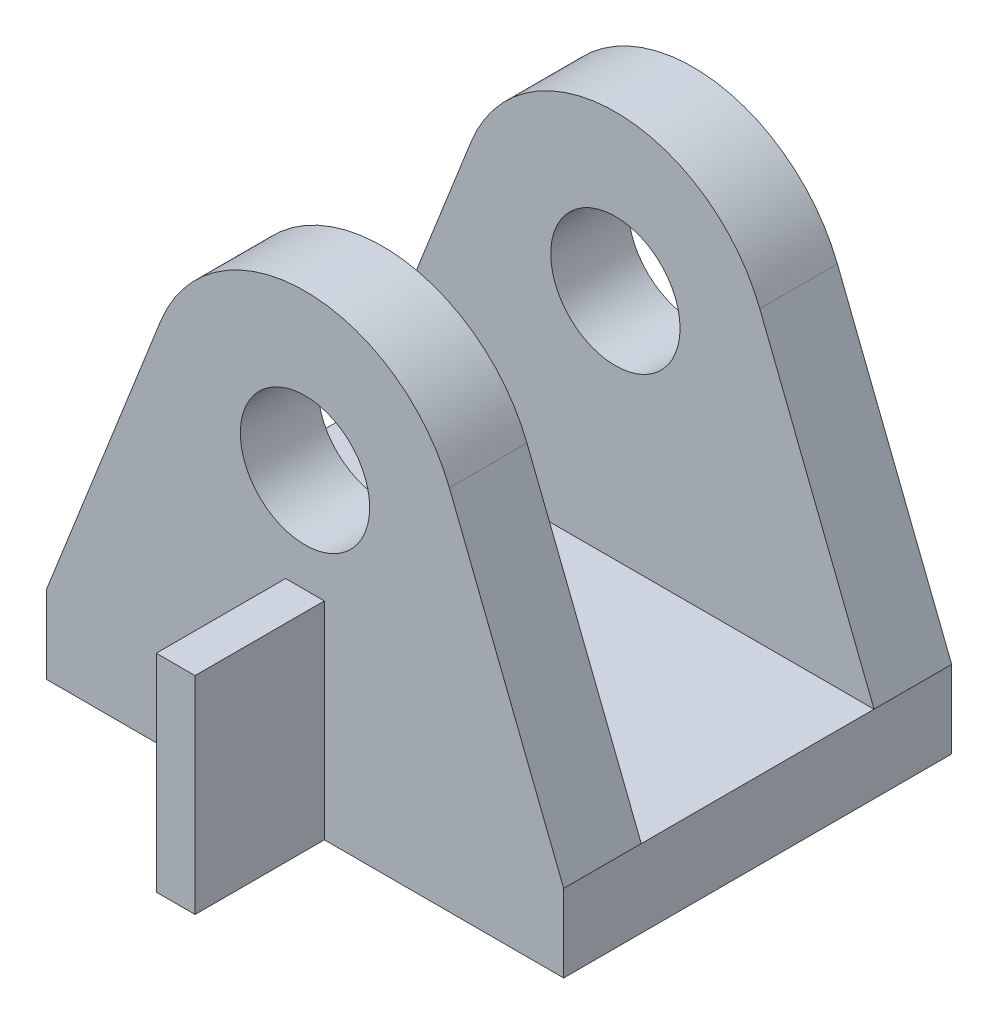
from build123d import *

# Parameters (mm, degrees)
SKETCH_1_W           = 200
SKETCH_1_H           = 150
BOSS_EXTRUDE_1_DEPTH = 30
SKETCH_2_R           = 25
BOSS_EXTRUDE_2_DEPTH = 30
SKETCH_4_W           = 15
SKETCH_4_H           = 80
BOSS_EXTRUDE_3_DEPTH = 50


with BuildPart() as part:
    # Sketch 1 → Boss-Extrude 1 (new body)
    with BuildSketch(Plane(origin=(0, 0, 0), x_dir=(1, 0, 0), z_dir=(0, 1, 0))):
        Rectangle(SKETCH_1_W, SKETCH_1_H)
    extrude(amount=BOSS_EXTRUDE_1_DEPTH)

    # Sketch 2 → Boss-Extrude 2 (add)
    with BuildSketch(Plane.XY.offset(75)):
        with BuildLine():
            Line((-55.814702058, 142.01633562), (-100, 30))
            Line((-100, 30), (100, 30))
            Line((100, 30), (55.814702058, 142.01633562))
            ThreePointArc((55.814702058, 142.01633562), (0, 180), (-55.814702058, 142.01633562))
        make_face()
        with Locations((0, 120)):
            Circle(SKETCH_2_R, mode=Mode.SUBTRACT)
    boss_extrude_2 = extrude(amount=-BOSS_EXTRUDE_2_DEPTH)

    # Sketch 4 → Boss-Extrude 3 (add)
    with BuildSketch(Plane.XY.offset(75)):
        with Locations((0, 40)):
            Rectangle(SKETCH_4_W, SKETCH_4_H)
    boss_extrude_3 = extrude(amount=BOSS_EXTRUDE_3_DEPTH)

    # Mirror 1: Boss-Extrude 2, Boss-Extrude 3 across plane
    add(boss_extrude_2.mirror(Plane.XY))
    add(boss_extrude_3.mirror(Plane.XY))


solid = part.part
